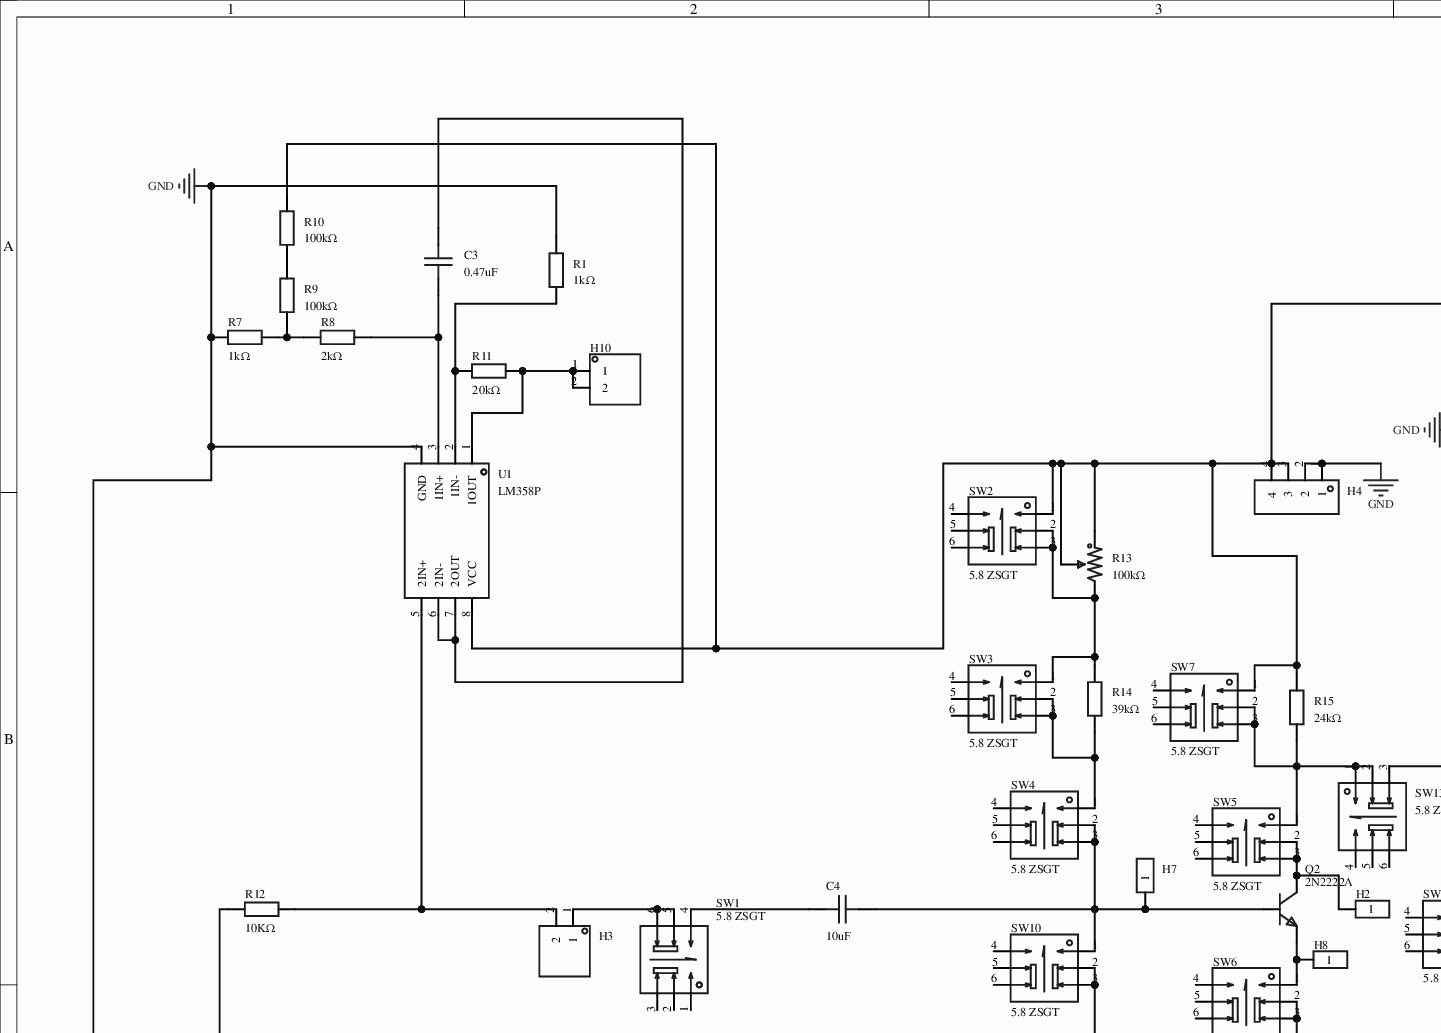
[diagram p0: MISC52134-3.schdoc, top left]
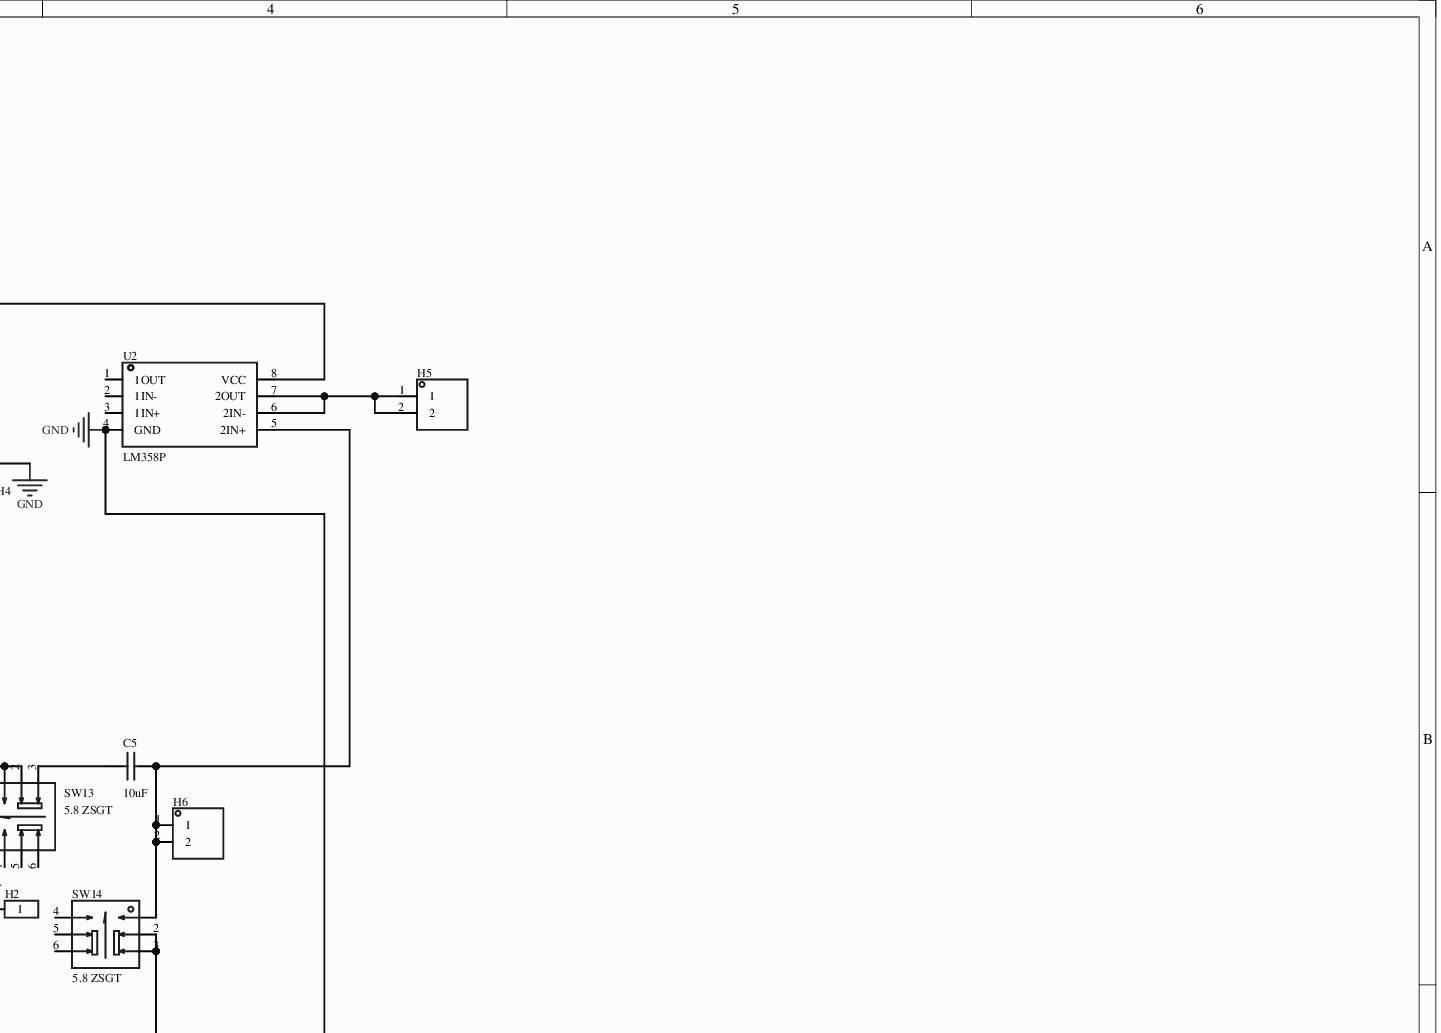
[diagram p1: MISC52134-3.schdoc, top right]
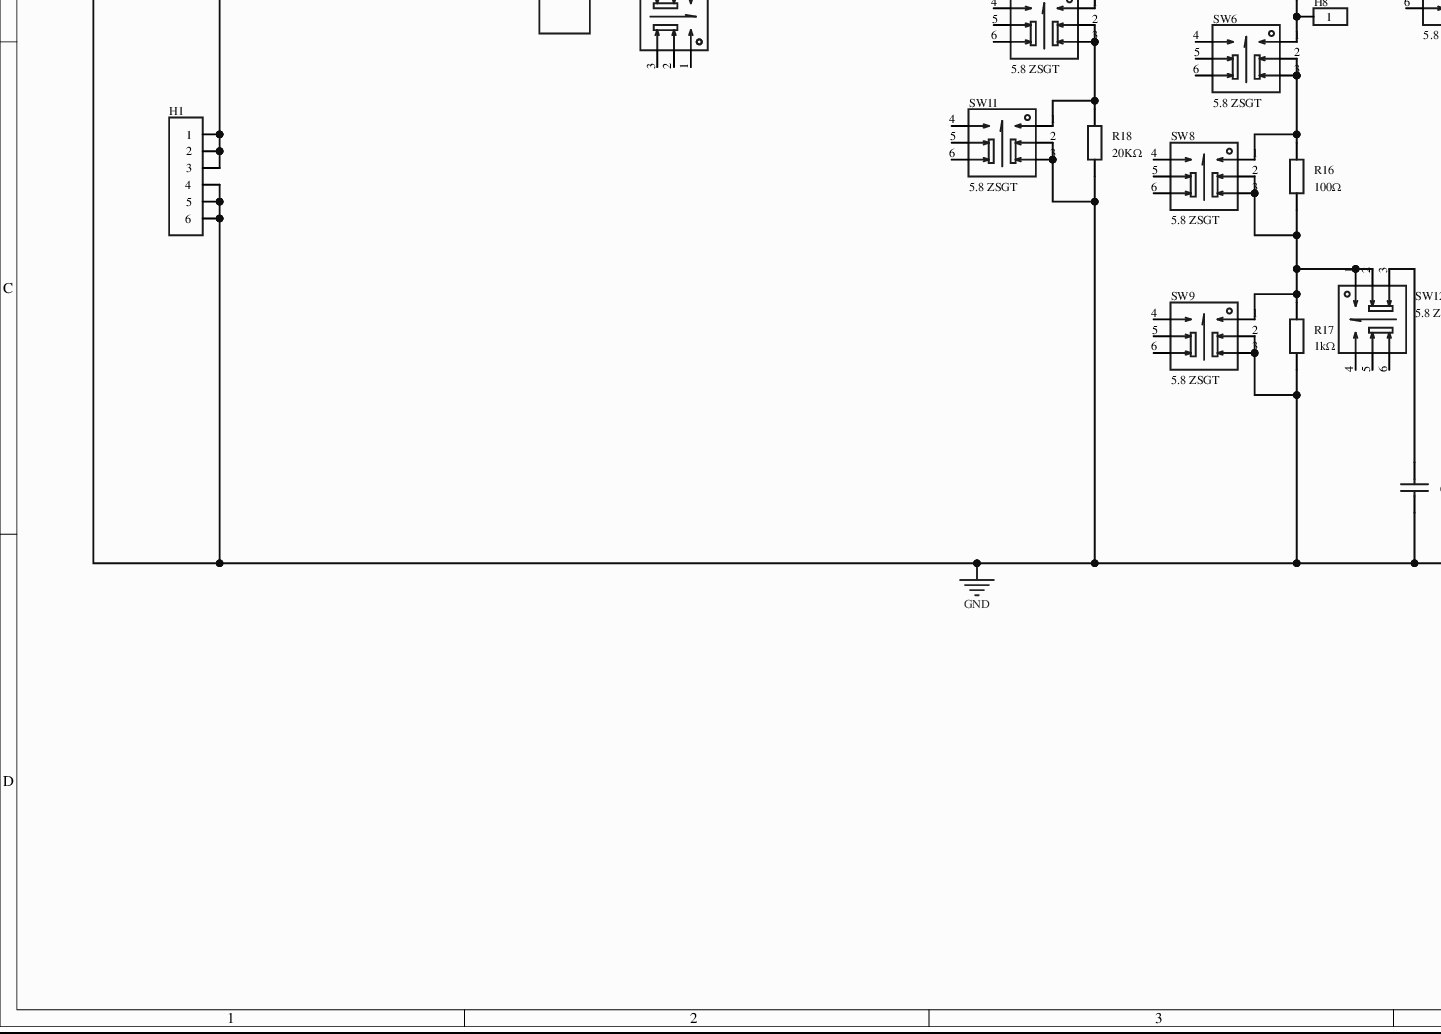
[diagram p2: MISC52134-3.schdoc, bottom left]
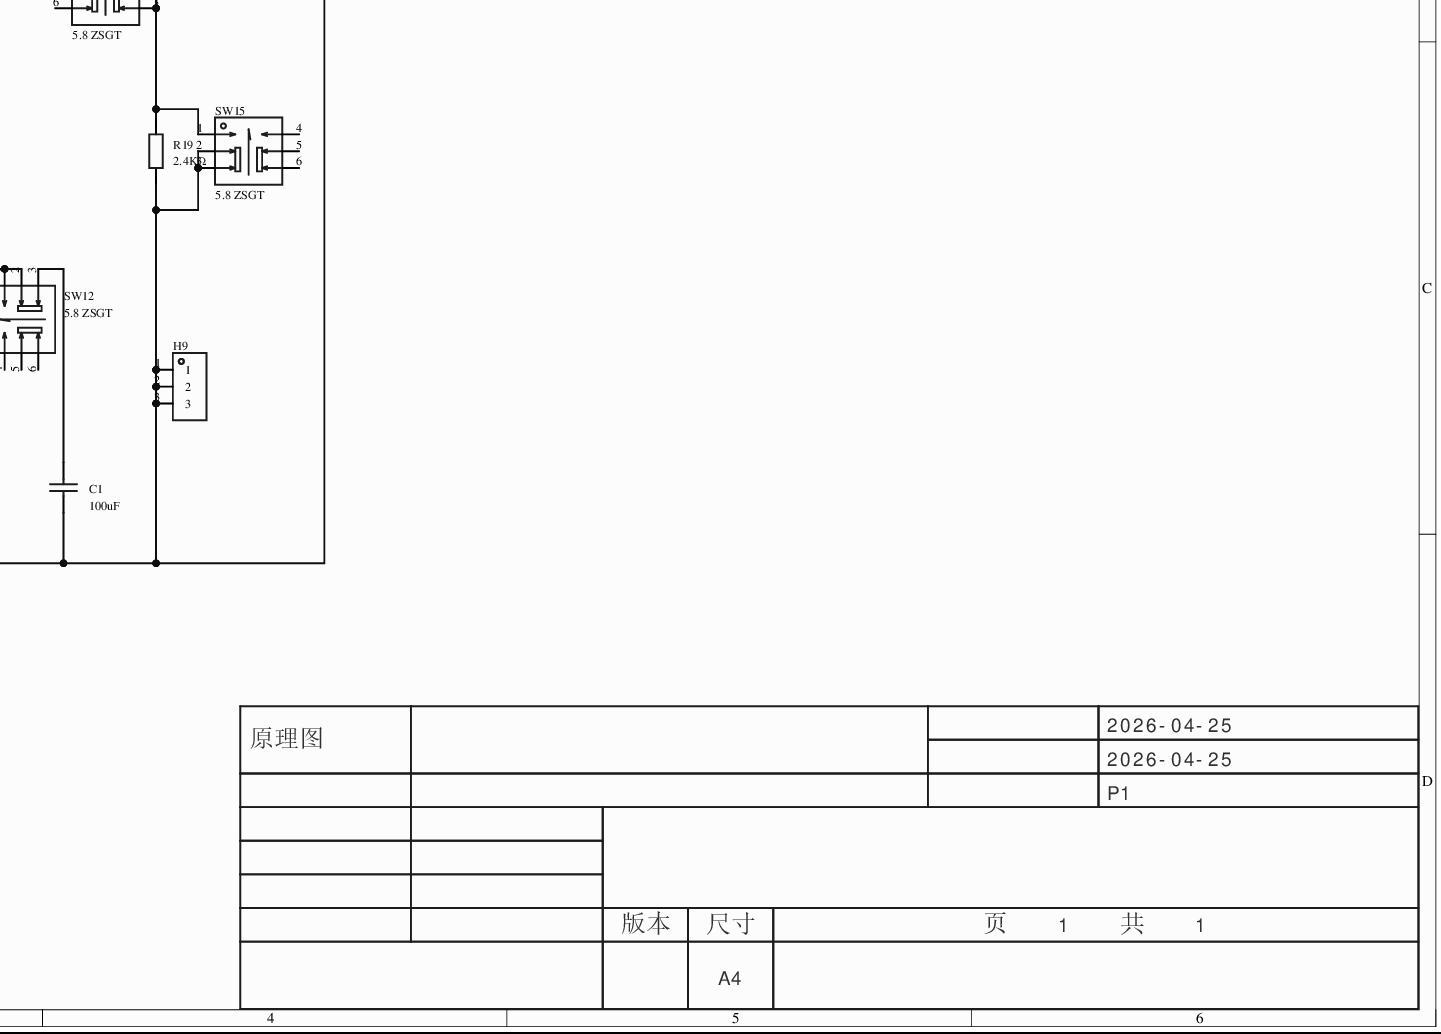
[diagram p3: MISC52134-3.schdoc, bottom right]
# Altium project MISC52134-2.PrjPcb
1 sheet, 46 parts. Net scope: global (net labels, ports and power ports of the same name join across sheets).
Board file: MISC52134.pcbdoc

## Sheet MISC52134-3.schdoc
size 420 x 297 mm; Version: V1.0; @Project Name: MISC52134; @Update Date: 2026-04-25; @Create Date: 2026-04-25; @Board Name: MISC52134; @Create Time: 23:31:58; @Page Count: 1; @Page No: 1; @Schematic Name: MISC52134; @Update Time: 23:31:58; Size: A4

### Parts
C1  100uF  [C0805]
C3  0.47uF  [C0603]
C4  10uF  [C0603]
C5  10uF  [C0805]
H1  (no value)  [HDR-TH_6P-P2.54-V-M-1]
H2  (no value)  [HDR-TH_1P-V-M_XKB_X4611WV-01I-C28D40]
H3  (no value)  [HDR-TH_2P-P2.54-V-M-1]
H4  (no value)  [HDR-TH_4P-P2.54-V-M]
H5  (no value)  [HDR-TH_2P-P2.54-V-M-1]
H6  (no value)  [HDR-TH_2P-P2.54-V-M-1]
H7  (no value)  [HDR-TH_1P-V-M_XKB_X4611WV-01I-C28D40]
H8  (no value)  [HDR-TH_1P-V-M_XKB_X4611WV-01I-C28D40]
H9  (no value)  [HDR-TH_3P-P2.54-V-M]
H10  (no value)  [HDR-TH_2P-P2.54-V-M-1]
Q2  2N2222A  [TO-92-3_L4.9-W3.7-P1.27-L]
R1  1kΩ  [R0603]
R7  1kΩ  [R0603]
R8  2kΩ  [R0603]
R9  100kΩ  [R0603]
R10  100kΩ  [R0603]
R11  20kΩ  [R0603]
R12  10KΩ  [R0603]
R13  100kΩ  [RES-ADJ-SMD_JER33X-1-14]
R14  39kΩ  [R0603]
R15  24kΩ  [R0603]
R16  100Ω  [R0603]
R17  1kΩ  [R0603]
R18  20KΩ  [R0603]
R19  2.4KΩ  [R0603]
SW1  5.8 ZSGT  [SW-TH_5.8ZSGT]
SW2  5.8 ZSGT  [SW-TH_5.8ZSGT]
SW3  5.8 ZSGT  [SW-TH_5.8ZSGT]
SW4  5.8 ZSGT  [SW-TH_5.8ZSGT]
SW5  5.8 ZSGT  [SW-TH_5.8ZSGT]
SW6  5.8 ZSGT  [SW-TH_5.8ZSGT]
SW7  5.8 ZSGT  [SW-TH_5.8ZSGT]
SW8  5.8 ZSGT  [SW-TH_5.8ZSGT]
SW9  5.8 ZSGT  [SW-TH_5.8ZSGT]
SW10  5.8 ZSGT  [SW-TH_5.8ZSGT]
SW11  5.8 ZSGT  [SW-TH_5.8ZSGT]
SW12  5.8 ZSGT  [SW-TH_5.8ZSGT]
SW13  5.8 ZSGT  [SW-TH_5.8ZSGT]
SW14  5.8 ZSGT  [SW-TH_5.8ZSGT]
SW15  5.8 ZSGT  [SW-TH_5.8ZSGT]
U1  LM358P  [DIP-8_L9.4-W6.4-P2.54-LS9.1-BL]
U2  LM358P  [DIP-8_L9.4-W6.4-P2.54-LS9.1-BL]

### Nets
GND: C1.1 H1.4 H1.5 H1.6 H4.1 H4.2 H9.1 H9.2 H9.3 R1.2 R7.1 R17.1 R18.1 R19.1 SW9.2 SW9.3 SW11.2 SW11.3 SW15.2 SW15.3 U1.4(GND) U2.4(GND)
NetC1_2: C1.2 SW12.3
NetC3_1: C3.1 R8.2 U1.3(1IN+)
NetC3_2: C3.2 U1.6(2IN-) U1.7(2OUT)
NetC4_1: C4.1 SW1.4
NetC4_2: C4.2 H7.1 Q2.2(B) SW4.2 SW4.3 SW10.1
NetC5_1: C5.1 H6.1 H6.2 SW14.1 U2.5(2IN+)
NetC5_2: C5.2 SW13.3
NetH1_1: H1.1 H1.2 H1.3 R12.1
NetH2_1: H2.1 Q2.3(C) SW5.2 SW5.3
NetH3_1: H3.1 SW1.5 SW1.6
NetH3_2: H3.2 R12.2 U1.5(2IN+)
NetH4_3: H4.3 H4.4 R10.2 R13.1 R13.2 R15.2 SW2.1 SW7.1 U1.8(VCC) U2.8(VCC)
NetH5_1: H5.1 H5.2 U2.6(2IN-) U2.7(2OUT)
NetH8_1: H8.1 Q2.1(E) SW6.1
NetH10_1: H10.1 H10.2 R11.2 U1.1(1OUT)
NetR1_1: R1.1 R11.1 U1.2(1IN-)
NetR7_2: R7.2 R8.1 R9.1
NetR9_2: R9.2 R10.1
NetR13_3: R13.3 R14.2 SW2.2 SW2.3 SW3.1
NetR14_1: R14.1 SW3.2 SW3.3 SW4.1
NetR15_1: R15.1 SW5.1 SW7.2 SW7.3 SW13.1 SW13.2
NetR16_1: R16.1 R17.2 SW8.2 SW8.3 SW9.1 SW12.1 SW12.2
NetR16_2: R16.2 SW6.2 SW6.3 SW8.1
NetR18_2: R18.2 SW10.2 SW10.3 SW11.1
NetR19_2: R19.2 SW14.2 SW14.3 SW15.1

Not connected (* = marked no-connect by the designer): SW1 1 2 3; SW2 4 5 6; SW3 4 5 6; SW4 4 5 6; SW5 4 5 6; SW6 4 5 6; SW7 4 5 6; SW8 4 5 6; SW9 4 5 6; SW10 4 5 6; SW11 4 5 6; SW12 4 5 6; SW13 4 5 6; SW14 4 5 6; SW15 4 5 6; U2 1(1OUT) 2(1IN-) 3(1IN+)

### Notes on the sheet
- 2026-04-25
- 原理图
- P1
- 版本
- 尺寸
- A4
- 页    1    共    1

### Library data of the parts
C1 C5 = GRM21BR60J107ME15L: 容值:100uF;精度:±20%;额定电压:6.3V;温度系数:X5R;; Manufacturer: muRata(村田); AddInBom: yes; ModelId: 1ba041120af144c991958decab20d2410819f05c4eef4c71ace90d822a990e87; ModelName: C0805_L2.0-W1.3-H1.3; ModelTransform: 78.74,51.181,0,0,0,0,0,0.0005,0; Tolerance: ±20%; Voltage Rating: 6.3V; Temperature Coefficient: X5R; Symbol: GRM21BR60J107ME15L; Device: GRM21BR60J107ME15L; LCSC Part Name: 100uF ±20% 6.3V; ManufacturerPart: GRM21BR60J107ME15L; Supplier Footprint: 0805; JLCPCB Part Class: Extended Part; Datasheet: https://item.szlcsc.com/datasheet/GRM21BR60J107ME15L/152991.html; Supplier: LCSC; ConvertToPcb: yes; FootprintName: C0805
  C1: SupplierPart: C141660; Value: 100uF
  C5: Value: 10uF
C3 C4 = CGA0603X5R106K100JT: 容值:10uF;精度:±10%;额定电压:10V;温度系数:X5R;; Manufacturer: HRE(芯声); AddInBom: yes; ModelId: ac125912035d415993ca9572d50418b10819f05c4eef4c71ace90d822a990e87; ModelName: C0603_L1.6-W0.8-H0.8; ModelTransform: 62.992,31.496,0,0,0,0,0,0,0; Tolerance: ±10%; Voltage Rating: 10V; Temperature Coefficient: X5R; Symbol: CGA0603X5R106K100JT; Device: CGA0603X5R106K100JT; LCSC Part Name: 10uF ±10% 10V; ManufacturerPart: CGA0603X5R106K100JT; Supplier Footprint: 0603; JLCPCB Part Class: Extended Part; Datasheet: https://item.szlcsc.com/datasheet/CGA0603X5R106K100JT/7062548.html; Supplier: LCSC; ConvertToPcb: yes; FootprintName: C0603
  C3: Value: 0.47uF
  C4: SupplierPart: C6119842; Value: 10uF
H1 = HDR-M_2.54_1x6P: Symbol: Header-Male-2.54_1x6; ConvertToPcb: yes; ModelId: 60739dffc9b04830a286435b0fefbd4a0819f05c4eef4c71ace90d822a990e87; ModelName: HDR2.54-M-LI-1X6P; ModelTransform: 599.999,100,0,0,0,0,0,0,-118.11; Device: HDR-M_2.54_1x6P; AddInBom: yes; SupplierPart: C37208; Supplier Footprint: 插件; FootprintName: HDR-TH_6P-P2.54-V-M-1
H2 H7 H8 = HDR-M_2.54_1x1P: Symbol: HDR_1x1; ConvertToPcb: yes; ModelId: 95857080d3cc4057a19a22ccce05e1710819f05c4eef4c71ace90d822a990e87; ModelTransform: 78.74,79.1337,0,0,0,0,0,0,-110.236; Device: HDR-M_2.54_1x1P; AddInBom: yes; SupplierPart: C81276; Supplier Footprint: 插件; FootprintName: HDR-TH_1P-V-M_XKB_X4611WV-01I-C28D40; JLCPCB Part Class: Extended Part; ModelName: HDR-TH_1P-V-M_XKB_X4611WV-01I-C28D40
H3 H5 H6 H10 = HDR-M_2.54_1x2P: Symbol: 210S-1*2P L=11.6MMGold-plated black; ConvertToPcb: yes; ModelId: 79b2e9f2d70a4d68a1b7098f27c6d4c50819f05c4eef4c71ace90d822a990e87; ModelName: HDR-M-2.54_1x2; ModelTransform: 200,100,0,0,0,0,0,0,-118.11; Device: HDR-M_2.54_1x2P; AddInBom: yes; SupplierPart: C124375; Supplier Footprint: 插件; FootprintName: HDR-TH_2P-P2.54-V-M-1
H4 = HDR-M_2.54_1x4P: Symbol: PZ254V-11-04P; ConvertToPcb: yes; ModelId: 112f4d05e8d64e99ab9a333894bea4f90819f05c4eef4c71ace90d822a990e87; ModelName: HDR-TH_4P-P2.54-M-LI-1X4P; ModelTransform: 399.999,104.7242,0,0,0,0,0,0,-118.11; Device: HDR-M_2.54_1x4P; AddInBom: yes; SupplierPart: C492403; Supplier Footprint: 插件; FootprintName: HDR-TH_4P-P2.54-V-M
H9 = HDR-M_2.54_1x3P: AddInBom: yes; ModelId: bb473b6d38ff42a99216a4fcdbdcc4cb0819f05c4eef4c71ace90d822a990e87; ModelName: HDR-TH_3P-P2.54-M-LI-1X3P; ModelTransform: 300.03877,100,0,0,0,0,0,0,-118.11; Symbol: HDR-M_2.54_1x3P; Device: HDR-M_2.54_1x3P; ConvertToPcb: yes; FootprintName: HDR-TH_3P-P2.54-V-M; SupplierPart: C2937625; Supplier Footprint: 插件
Q2 = 2N2222A: 晶体管类型:NPN;集电极电流(Ic):600mA;集射极击穿电压(Vceo):40V;耗散功率(Pd):625mW;直流电流增益(hFE):40@500mA,10V;; Manufacturer: ST(先科); Symbol: 2N2222(Sim); AddInBom: yes; ModelId: aafe8e06f2154e7c93506efd0d6632dd0819f05c4eef4c71ace90d822a990e87; ModelTransform: 176.28752,144.88554,0,180,0,0,0,20.669,-196.85; type: NPN; Current - Collector(Ic): 600mA; Collector - Emitter Voltage VCEO: 40V; Pd - Power Dissipation: 625mW; Transition frequency(fT): 250MHz; Current - Collector Cutoff: 10nA; Vce Saturation(VCE(sat)): 1V; Emitter-Base Voltage(Vebo): 6V; Number: 1个NPN; Device: 2N2222A; LCSC Part Name: NPN 电流:600mA 电压:40V; SupplierPart: C118536; ManufacturerPart: 2N2222A; Supplier Footprint: TO-92; JLCPCB Part Class: Extended Part; Datasheet: https://item.szlcsc.com/datasheet/2N2222A/119803.html; Supplier: LCSC; ConvertToPcb: yes; FootprintName: TO-92-3_L4.9-W3.7-P1.27-L; ModelName: TO-92-3_L4.9-W3.7-P1.27-L; DC Current Gain: 40@500mA,10V; Operating Temperature: -
R1 R7-R11 = 0603WAF1001T5E: 电阻类型:厚膜电阻;阻值:1kΩ;精度:±1%;功率:100mW;工作电压:75V;温度系数:±100ppm/℃;; Manufacturer: UNI-ROYAL(厚声); AddInBom: yes; ModelId: fc143cca1e79419f9cd78b61e9279f080819f05c4eef4c71ace90d822a990e87; ModelTransform: 31.8897,63.7794,0,90,0,0,0,0,0; Tolerance: ±1%; Power(Watts): 100mW; Voltage-Supply(Max): 75V; Symbol: 0603WAF1001T5E; Device: 0603WAF1001T5E; LCSC Part Name: 1kΩ ±1% 100mW 厚膜电阻; ManufacturerPart: 0603WAF1001T5E; Supplier Footprint: 0603; JLCPCB Part Class: Basic Part; Datasheet: https://item.szlcsc.com/datasheet/0603WAF1001T5E/21904.html; Supplier: LCSC; ConvertToPcb: yes; FootprintName: R0603; ModelName: R0603; Type: 厚膜电阻; Temperature Coefficient: ±100ppm/℃; Operating Temperature: -55℃~+155℃
  R1 R7: SupplierPart: C21190; Value: 1kΩ
  R8: Value: 2kΩ
  R9 R10: Value: 100kΩ
  R11: Value: 20kΩ
R12 = RC0603FR-07100RL: 电阻类型:厚膜电阻;阻值:100Ω;精度:±1%;功率:100mW;最大工作电压:75V;温度系数:±100ppm/℃;; Manufacturer: YAGEO(国巨); AddInBom: yes; ModelId: fc143cca1e79419f9cd78b61e9279f080819f05c4eef4c71ace90d822a990e87; ModelTransform: 31.8897,63.7794,0,90,0,0,0,0,0; Tolerance: ±1%; Power(Watts): 100mW; Overload Voltage (Max): 75V; Symbol: RC0603FR-07100RL; Device: RC0603FR-07100RL; Value: 10KΩ; LCSC Part Name: 厚膜电阻 100Ω ±1% 100mW; ManufacturerPart: RC0603FR-07100RL; Supplier Footprint: 0603; JLCPCB Part Class: Extended Part; Datasheet: https://atta.szlcsc.com/upload/public/pdf/source/20180316/70C0E2BDAE7FCC62C531A5A58D202EE1.pdf; Supplier: LCSC; ConvertToPcb: yes; FootprintName: R0603; ModelName: R0603; Type: 厚膜电阻; Temperature Coefficient: ±100ppm/℃; Operating Temperature Range: -55℃~+155℃
R13 = JER33X-1-15: 阻值:100kΩ;精度:±25%;功率:150mW;温度系数:±250ppm/℃;; Manufacturer: JIERR(捷而瑞); AddInBom: yes; ModelId: de65341884c4454393239133889d31970819f05c4eef4c71ace90d822a990e87; ModelTransform: 120.4722,150,0,0,0,0,0,0,0; Tolerance: ±25%; Power(Watts): 150mW; Number of Turns: 1; Symbol: JER33X-1-15; Device: JER33X-1-15; LCSC Part Name: 玻璃釉贴片电位器; SupplierPart: C48997895; ManufacturerPart: JER33X-1-15; Supplier Footprint: SMD-3P,3.4x3.1mm; JLCPCB Part Class: Extended Part; Datasheet: https://item.szlcsc.com/datasheet/JER33X-1-15/51342031.html; Supplier: LCSC; ConvertToPcb: yes; FootprintName: RES-ADJ-SMD_JER33X-1-14; ModelName: RES-ADJ-SMD_JER33X-1-14; Value: 100kΩ; Temperature Coefficient: ±250ppm/℃
R14-R19 = 0603WAF3902T5E: 电阻类型:厚膜电阻;阻值:39kΩ;精度:±1%;功率:100mW;最大工作电压:75V;温度系数:±100ppm/℃;; Manufacturer: UNI-ROYAL(厚声); AddInBom: yes; ModelId: fc143cca1e79419f9cd78b61e9279f080819f05c4eef4c71ace90d822a990e87; ModelTransform: 31.8897,63.7794,0,90,0,0,0,0,0; Tolerance: ±1%; Power(Watts): 100mW; Overload Voltage (Max): 75V; Symbol: 0603WAF3902T5E; Device: 0603WAF3902T5E; LCSC Part Name: 39kΩ ±1% 100mW 厚膜电阻; ManufacturerPart: 0603WAF3902T5E; Supplier Footprint: 0603; JLCPCB Part Class: Basic Part; Datasheet: https://atta.szlcsc.com/upload/public/pdf/source/20200306/C422600_1E6D84923E4A46A82E41ADD87F860B5C.pdf; Supplier: LCSC; ConvertToPcb: yes; FootprintName: R0603; ModelName: R0603; Type: 厚膜电阻; Temperature Coefficient: ±100ppm/℃; Operating Temperature Range: -55℃~+155℃
  R14: Value: 39kΩ
  R15: Value: 24kΩ
  R16: Value: 100Ω
  R17: Value: 1kΩ
  R18: Value: 20KΩ
  R19: Value: 2.4KΩ
SW1-SW15 = 5.8 ZSGT: 电路结构:双刀双掷;自锁/无锁:自锁;安装方式:直插;触点电流:110mA;额定电压:30V;带灯:不带;作用力:1.5N;工作寿命:10万次;; Manufacturer: SHOU HAN(首韩); AddInBom: yes; ModelId: 3b6e980975cd43bda015b2e9aaa869d30819f05c4eef4c71ace90d822a990e87; ModelTransform: 228.346,228.346,0,0,0,0,0,0,-141.732; Circuit: 双刀双掷; Self Lock / No Lock: 自锁; Actuator Style: 方形按钮; Contact Current: 110mA; Voltage Rating: 30V; Actuator/Cap Color: 白色; With Lamp: 不带; Operating Force: 1.5N; Life: 10万次; Symbol: 5.8 ZSGT; Device: 5.8 ZSGT; LCSC Part Name: 5.8*5.8有头/高头 带锁/自锁开关 泡泡机开关; SupplierPart: C2681587; ManufacturerPart: 5.8 ZSGT; Supplier Footprint: 插件; JLCPCB Part Class: Extended Part; Datasheet: https://item.szlcsc.com/datasheet/5.8%2520ZSGT/2774930.html; Supplier: LCSC; ConvertToPcb: yes; FootprintName: SW-TH_5.8ZSGT; ModelName: SW-TH_5.8ZSGT; Mounting Type: 直插; Termination Style: PC引脚; Operating Temperature: -10℃~+70℃
U1 U2 = LM358P: 放大器数:双路;轨到轨:-;增益带宽积(GBP):-;输入失调电压(Vos):3mV;压摆率(SR):300V/ms;输入偏置电流(Ib):20nA;; Manufacturer: TI(德州仪器); AddInBom: yes; ModelId: 5746b540d01a4d1b9eb6b4f989297bc70819f05c4eef4c71ace90d822a990e87; ModelName: DIP-8_L9.8-W6.6-H3.5-LS7.62-P2.54; ModelTransform: 385.826,311.8104,0,0,0,0,0,-0.0005,-118.11; Number of Channels: 双路; Maximum Power Supply Range (Vdd-Vss): 32V; Vos - Input Offset Voltage: 3mV; Input Offset Voltage Drift(Vos TC): 7uV/℃; Ib - Input Bias Current: 20nA; Noise density(eN): 40nV/√Hz@1kHz; Common Mode Rejection Ratio(CMRR): 80dB; Single supply: 3V~32V; Dual Supply: 1.5V~16V；-16V~-1.5V; Symbol: LM358P; Device: LM358P; LCSC Part Name: 双通道运算放大器; SupplierPart: C5213; ManufacturerPart: LM358P; Supplier Footprint: DIP-8; JLCPCB Part Class: Extended Part; Datasheet: http://www.ti.com/cn/lit/gpn/lm358; Supplier: LCSC; ConvertToPcb: yes; FootprintName: DIP-8_L9.4-W6.4-P2.54-LS9.1-BL; Rail to Rail: -; Gain Bandwidth Product: -; Slew Rate: 300V/ms; Input Offset Current(Ios): -; Input offset current drift(Ios TC): -; Quiescent Current: -; Output Current: -; Operating Temperature: 0℃~+70℃